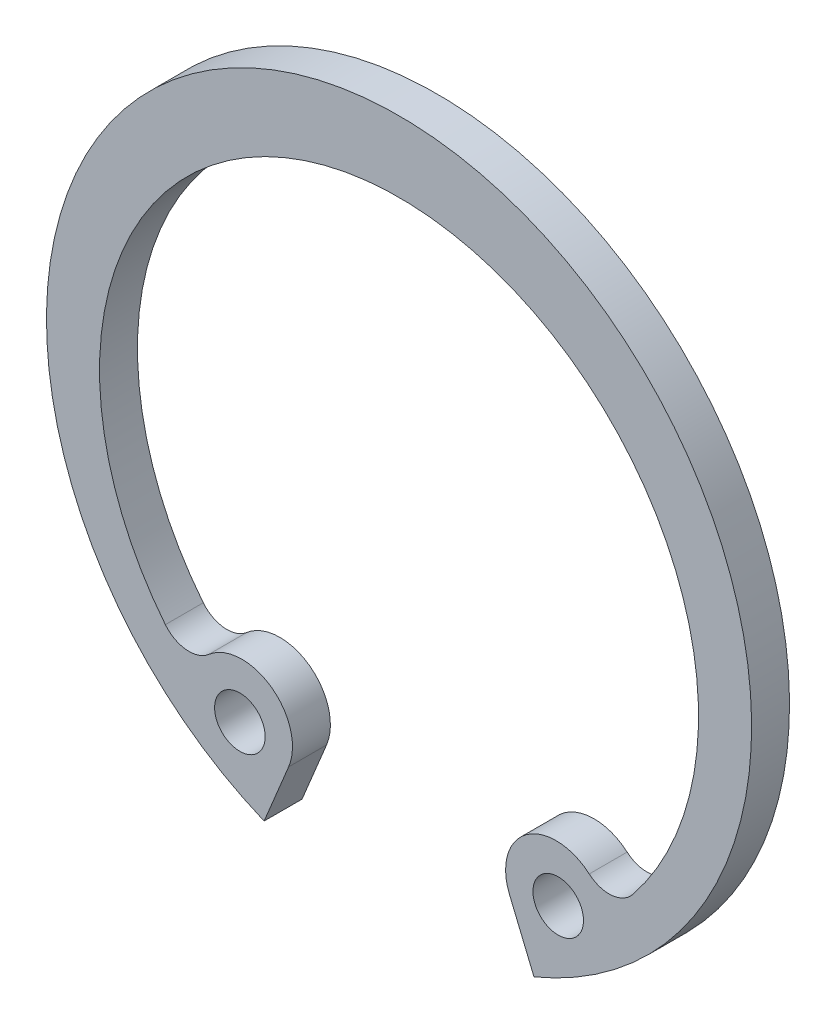
from build123d import *

# Parameters (mm, degrees)
SKETCH_1_R        = 1
EXTRUDE_967_DEPTH = 1.5


with BuildPart() as part:
    # 草图1 → Extrude 967 (new body)
    with BuildSketch(Plane.XY):
        with BuildLine():
            Line((-4.368765084, -10.547131916), (-5.338433881, -12.888119479))
            ThreePointArc((-5.338433881, -12.888119479), (0, 13.95), (5.338433881, -12.888119479))
            Line((5.338433881, -12.888119479), (4.368765084, -10.547131916))
            ThreePointArc((4.368765084, -10.547131916), (5.045920823, -8.160133818), (7.524722821, -8.268947735))
            ThreePointArc((7.524722821, -8.268947735), (8.418733826, -8.556288298), (9.245939718, -8.111821553))
            ThreePointArc((9.245939718, -8.111821553), (0, 11.15), (-9.245939718, -8.111821553))
            ThreePointArc((-9.245939718, -8.111821553), (-8.418733826, -8.556288298), (-7.524722821, -8.268947735))
            ThreePointArc((-7.524722821, -8.268947735), (-5.045920823, -8.160133818), (-4.368765084, -10.547131916))
        make_face()
        with Locations((-6.298089329, -9.978680815)):
            Circle(SKETCH_1_R, mode=Mode.SUBTRACT)
        with Locations(Location((6.298089329, -9.978680815, 0), (0, 0, 180))):
            Circle(SKETCH_1_R, mode=Mode.SUBTRACT)
    extrude(amount=EXTRUDE_967_DEPTH)


solid = part.part
